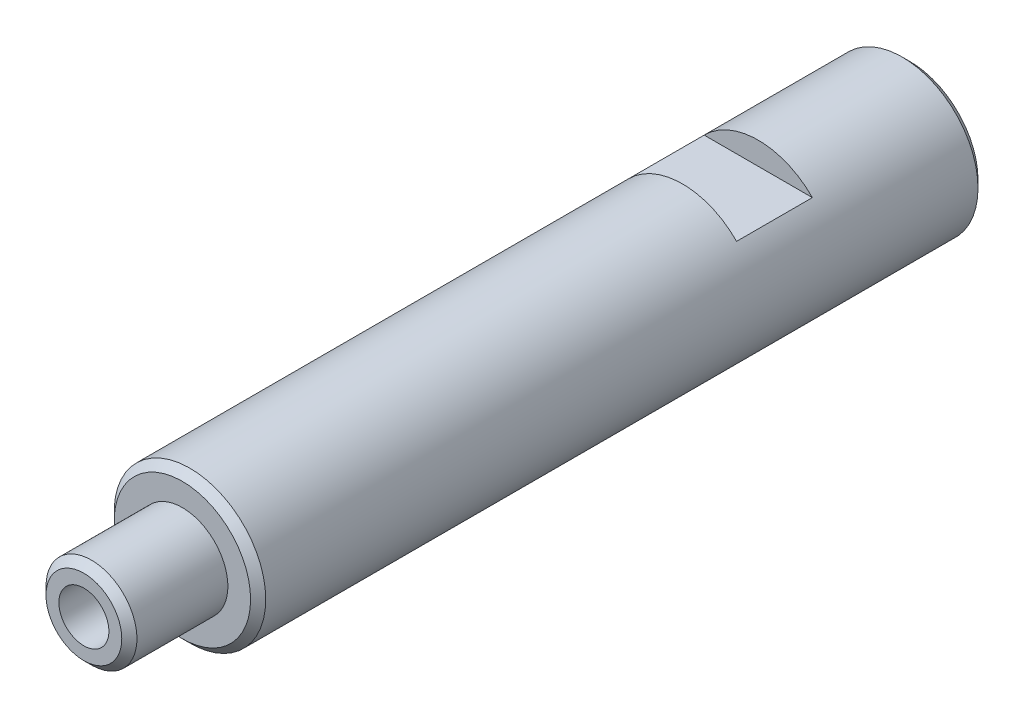
from build123d import *

# Parameters (mm, degrees)
SKETCH1_R             = 5
BOSS_EXTRUDE1_DEPTH   = 48
SKETCH2_R             = 3
BOSS_EXTRUDE2_DEPTH   = 6.5
M4_TAPPED_HOLE1_D     = 3.3
M4_TAPPED_HOLE1_DEPTH = 10.1
M4_TAPPED_HOLE1_TIP   = 0.991420021
M5_TAPPED_HOLE1_D     = 4.2
M5_TAPPED_HOLE1_DEPTH = 12.4
M5_TAPPED_HOLE1_TIP   = 1.2618073
CHAMFER1_SIZE         = 0.5
CUT_EXTRUDE1_START    = 5
SKETCH7_W             = 10
SKETCH7_H             = 5
CUT_EXTRUDE1_DEPTH    = 1.5


with BuildPart() as part:
    # Sketch1 → Boss-Extrude1 (new body)
    with BuildSketch(Plane.XY):
        Circle(SKETCH1_R)
    extrude(amount=BOSS_EXTRUDE1_DEPTH)

    # Sketch2 → Boss-Extrude2 (add)
    with BuildSketch(Plane.XY.offset(48)):
        with Locations(Location((0, 0, 0), (0, 0, 180))):
            Circle(SKETCH2_R)
    extrude(amount=BOSS_EXTRUDE2_DEPTH)

    # M4 Tapped Hole1
    with Locations(Plane.XY.offset(54.5)):
        with Locations((0, 0)):
            Hole(M4_TAPPED_HOLE1_D / 2, depth=M4_TAPPED_HOLE1_DEPTH)
            with Locations((0, 0, -(M4_TAPPED_HOLE1_DEPTH + M4_TAPPED_HOLE1_TIP / 2))):  # 118° drill point
                Cone(0, M4_TAPPED_HOLE1_D / 2, M4_TAPPED_HOLE1_TIP, mode=Mode.SUBTRACT)

    # M5 Tapped Hole1
    with Locations(Plane(origin=(0, 0, 0), x_dir=(-1, 0, 0), z_dir=(0, 0, -1))):
        with Locations((0, 0)):
            Hole(M5_TAPPED_HOLE1_D / 2, depth=M5_TAPPED_HOLE1_DEPTH)
            with Locations((0, 0, -(M5_TAPPED_HOLE1_DEPTH + M5_TAPPED_HOLE1_TIP / 2))):  # 118° drill point
                Cone(0, M5_TAPPED_HOLE1_D / 2, M5_TAPPED_HOLE1_TIP, mode=Mode.SUBTRACT)

    # Chamfer1
    chamfer1_edges = [part.edges().sort_by_distance(p)[0] for p in [
        (-5, 0, 0),
        (-5, 0, 48),
        (3, 0, 54.5),
    ]]
    chamfer(chamfer1_edges, length=CHAMFER1_SIZE)

    # Sketch7 → Cut-Extrude1 (cut, symmetric)
    with BuildSketch(Plane(origin=(0, 0, 0), x_dir=(1, 0, 0), z_dir=(0, 1, 0)).offset(CUT_EXTRUDE1_START)):
        with Locations((0, -12.5)):
            Rectangle(SKETCH7_W, SKETCH7_H)
    cut_extrude1 = extrude(amount=CUT_EXTRUDE1_DEPTH, both=True, mode=Mode.SUBTRACT)

    # Mirror1: Cut-Extrude1 across plane
    add(cut_extrude1.mirror(Plane.ZX), mode=Mode.SUBTRACT)


solid = part.part
